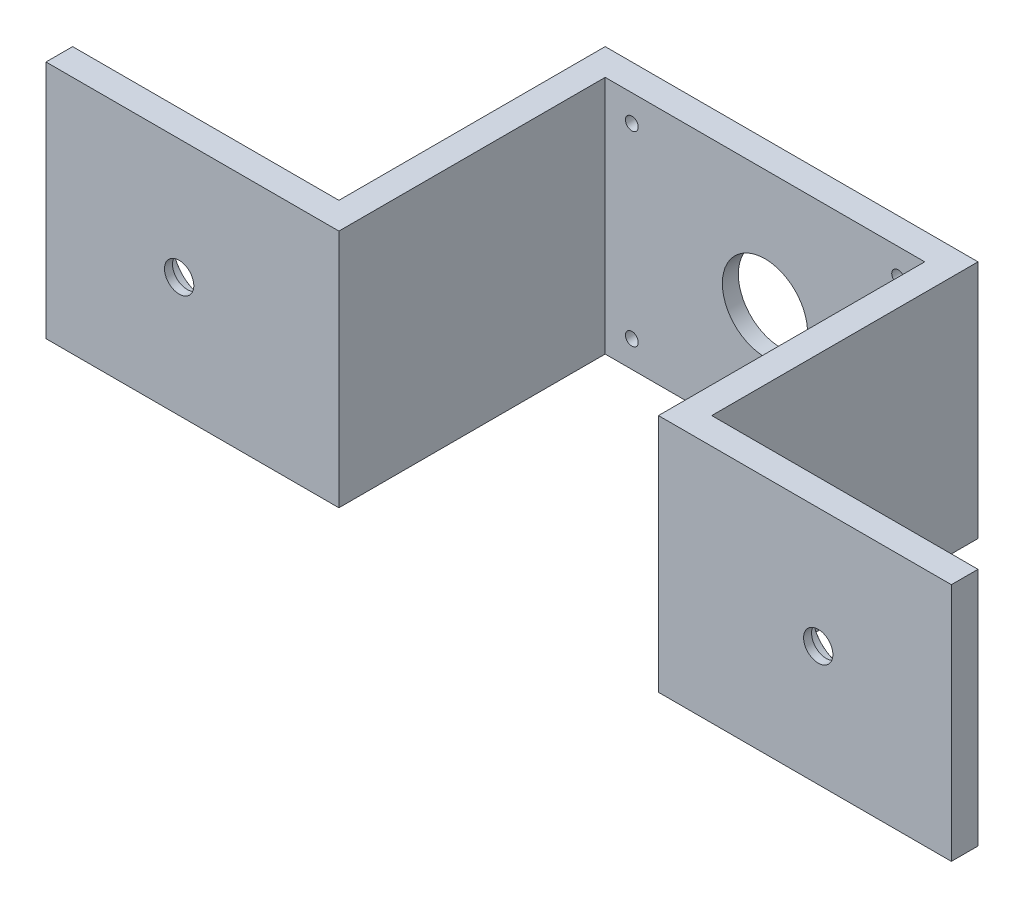
from build123d import *

# Parameters (mm, degrees)
BOSS_EXTRUDE3_DEPTH                    = 45
CBORE_FOR_M5_HEX_CAP_SCREW1_AT_2_COUNT = 2
CBORE_FOR_M5_HEX_CAP_SCREW1_AT_2_PITCH = 120
CUT_EXTRUDE1_DEPTH                     = 10
SKETCH13_R                             = 15
CUT_EXTRUDE2_DEPTH                     = 2
SKETCH14_R                             = 1.204328259
SKETCH14_R_2                           = 1.2
CUT_EXTRUDE3_DEPTH                     = 5


with BuildPart() as part:
    # Sketch7 → Boss-Extrude3 (new body)
    with BuildSketch(Plane(origin=(0, 0, 0), x_dir=(1, 0, 0), z_dir=(0, 1, 0))):
        Polygon((0, 0), (55, 0), (55, 50), (115, 50), (115, 0), (170, 0), (170, 5), (120, 5), (120, 55), (50, 55), (50, 5), (0, 5), align=None)
    extrude(amount=BOSS_EXTRUDE3_DEPTH)

    # Sketch10 → CBORE for M5 Hex Cap Screw1 (revolve, cut)
    with BuildSketch(Plane(origin=(145, 22.5, -5), x_dir=(0, 1, 0), z_dir=(1, 0, 0))):
        Polygon((0, 0), (0, 5), (2.75, 5), (2.75, 3.5), (6.119, 3.5), (6.119, 0.025), (6.144, 0), align=None)
    cbore_for_m5_hex_cap_screw1 = revolve(axis=Axis((145, 22.5, -11.35), (0, 0, 1)), mode=Mode.SUBTRACT)

    # CBORE for M5 Hex Cap Screw1 at 2: CBORE for M5 Hex Cap Screw1 ×2
    with Locations(*[(-i * CBORE_FOR_M5_HEX_CAP_SCREW1_AT_2_PITCH, 0, 0) for i in range(1, CBORE_FOR_M5_HEX_CAP_SCREW1_AT_2_COUNT)]):
        add(cbore_for_m5_hex_cap_screw1, mode=Mode.SUBTRACT)

    # Sketch12 → Cut-Extrude1 (cut)
    with BuildSketch(Plane(origin=(0, 0, -55), x_dir=(-1, 0, 0), z_dir=(0, 0, -1))):
        with BuildLine():
            ThreePointArc((-77, 22.5), (-82.745606781, 30.175787335), (-91.729427803, 26.826060731))
            Line((-91.729427803, 26.826060731), (-78.270572197, 18.173939269))
            ThreePointArc((-78.270572197, 18.173939269), (-77.324212665, 20.245606781), (-77, 22.5))
        make_face()
        with BuildLine():
            Line((-78.270572197, 18.173939269), (-91.729427803, 26.826060731))
            ThreePointArc((-91.729427803, 26.826060731), (-89.326060731, 15.770572197), (-78.270572197, 18.173939269))
        make_face()
    extrude(amount=-CUT_EXTRUDE1_DEPTH, mode=Mode.SUBTRACT)

    # Sketch13 → Cut-Extrude2 (cut)
    with BuildSketch(Plane(origin=(0, 0, -55), x_dir=(-1, 0, 0), z_dir=(0, 0, -1))):
        with Locations((-85, 22.5)):
            Circle(SKETCH13_R)
    extrude(amount=-CUT_EXTRUDE2_DEPTH, mode=Mode.SUBTRACT)

    # Sketch14 → Cut-Extrude3 (cut)
    with BuildSketch(Plane(origin=(0, 0, -55), x_dir=(-1, 0, 0), z_dir=(0, 0, -1))):
        with Locations((-60, 5)):
            Circle(SKETCH14_R)
        with Locations((-60, 40)):
            Circle(SKETCH14_R_2)
        with Locations((-110, 5)):
            Circle(SKETCH14_R_2)
        with Locations((-110, 40)):
            Circle(SKETCH14_R_2)
    extrude(amount=-CUT_EXTRUDE3_DEPTH, mode=Mode.SUBTRACT)


solid = part.part
